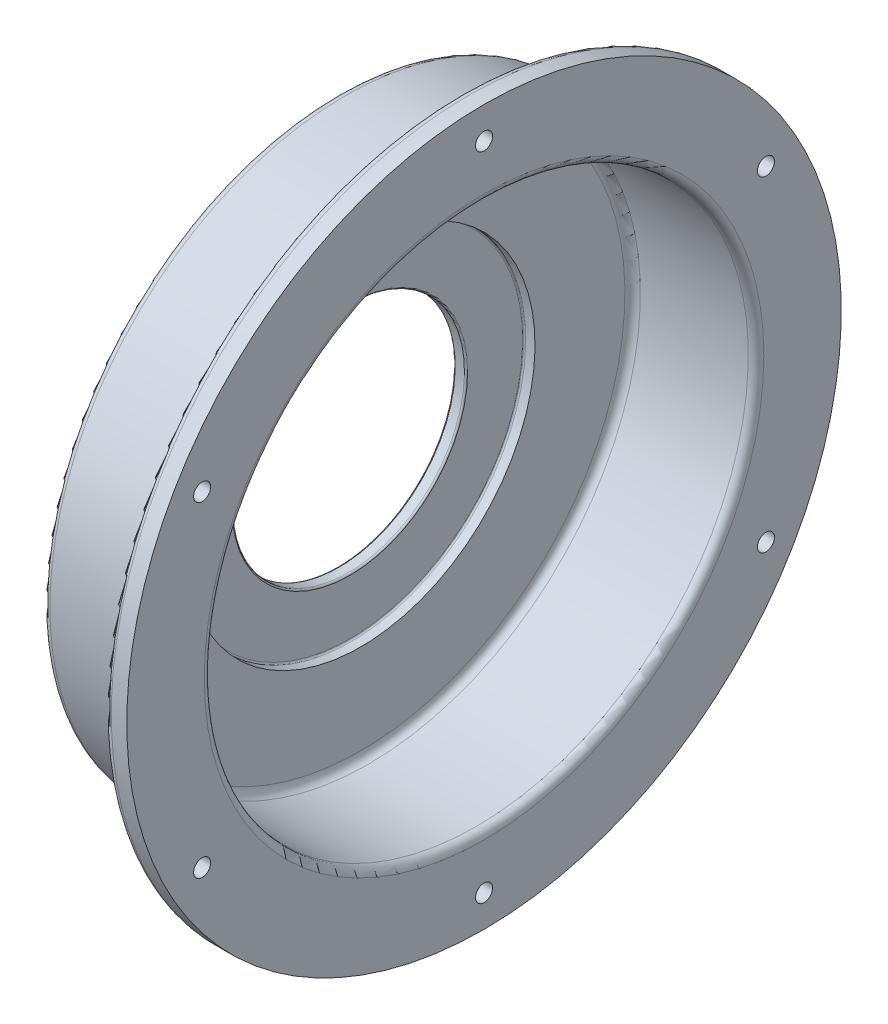
SolidWorks part; units mm, degrees
ref_plane "Front Plane" through (0, 0, 0) normal (0, 0, 1) x (1, 0, 0)
ref_plane "Top Plane" through (0, 0, 0) normal (0, 1, 0) x (1, 0, 0)
ref_plane "Right Plane" through (0, 0, 0) normal (1, 0, 0) x (0, 0, -1)
other "Configuration Table"
sketch "Sketch1" plane through (0, 0, 0) normal (0, 0, 1) x (1, 0, 0)
  line L0 (373.5199, 0) -> (11.1736, 0) construction
  line L1 (218.9199, 112.5) -> (212.9199, 112.5)
  line L2 (210.9199, 75) -> (204.9199, 75)
  line L3 (293.5199, 175.5) -> (223.9199, 175.5)
  line L4 (278.5199, 190.5) -> (208.9199, 190.5)
  line L5 (298.5199, 230.5) -> (298.5199, 205)
  line L6 (298.5199, 205) -> (298.5199, 180.5)
  line L7 (283.5199, 225.5) -> (283.5199, 195.5)
  line L8 (218.9199, 170.5) -> (218.9199, 131)
  line L9 (218.9199, 131) -> (218.9199, 112.5)
  line L10 (211.9199, 111.5) -> (211.9199, 76)
  line L11 (203.9199, 185.5) -> (203.9199, 131)
  line L12 (203.9199, 131) -> (203.9199, 76)
  line L13 (298.5199, 230.5) -> (288.5199, 230.5)
  arc A0 (293.5199, 175.5) -> (298.5199, 180.5) centre (293.5199, 180.5) ccw
  arc A1 (278.5199, 190.5) -> (283.5199, 195.5) centre (278.5199, 195.5) ccw
  arc A2 (288.5199, 230.5) -> (283.5199, 225.5) centre (288.5199, 225.5) ccw
  arc A3 (223.9199, 175.5) -> (218.9199, 170.5) centre (223.9199, 170.5) ccw
  arc A4 (210.9199, 75) -> (211.9199, 76) centre (210.9199, 76) ccw
  arc A5 (212.9199, 112.5) -> (211.9199, 111.5) centre (212.9199, 111.5) ccw
  arc A6 (203.9199, 76) -> (204.9199, 75) centre (204.9199, 76) ccw
  arc A7 (208.9199, 190.5) -> (203.9199, 185.5) centre (208.9199, 185.5) ccw
revolve "Revolve2" add sketch "Sketch1" angle 360 about L0
sketch "Sketch2" plane through (283.5199, 0, 0) normal (-1, 0, 0) x (0, 0, 1)
  circle A0 centre (0, 0) radius 210 construction
  circle A1 centre (0, 210) radius 5.5
  circle A2 centre (181.8653, 105) radius 5.5
  circle A3 centre (181.8653, -105) radius 5.5
  circle A4 centre (0, -210) radius 5.5
  circle A5 centre (-181.8653, -105) radius 5.5
  circle A6 centre (-181.8653, 105) radius 5.5
  point P17 (0, 0)
  dimension "D1" = 6
extrude "Cut-Extrude1" cut sketch "Sketch2" against normal blind 85
